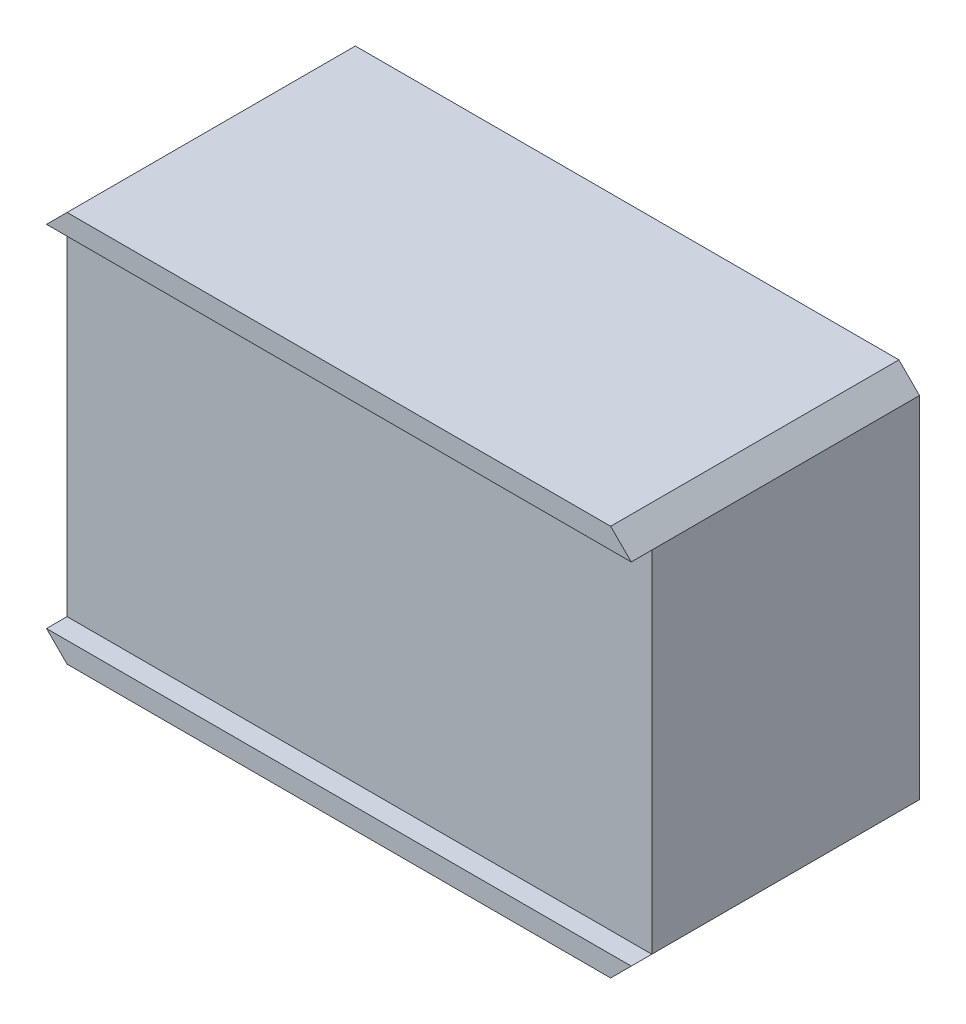
SolidWorks part; units mm, degrees
ref_plane "前视基准面" through (0, 0, 0) normal (0, 0, 1) x (1, 0, 0)
ref_plane "上视基准面" through (0, 0, 0) normal (0, 1, 0) x (1, 0, 0)
ref_plane "右视基准面" through (0, 0, 0) normal (1, 0, 0) x (0, 0, -1)
sketch "草图1" plane through (0, 0, 0) normal (0, 0, 1) x (1, 0, 0)
  line L1 (-28.4, -19) -> (28.4, -19)
  line L2 (-28.4, -19) -> (-28.4, 19)
  line L3 (-28.4, 19) -> (28.4, 19)
  line L4 (28.4, -19) -> (28.4, 19)
  line L5 (-28.4, -19) -> (28.4, 19) construction
  line L6 (-28.4, 19) -> (28.4, -19) construction
  point P0 (0, 0)
  dimension "D1" = 56.8
  dimension "D2" = 38
extrude "凸台-拉伸1" add sketch "草图1" along normal mid plane 28
chamfer "倒角1" distance 2 angle 45 4 edges at (28.4, -19, 0) (-28.4, -19, 0) (-28.4, 19, 0) (28.4, 19, 0)
sketch "草图2" plane through (28.4, 0, 0) normal (1, 0, 0) x (0, 0, -1)
  line L1 (-14, 17) -> (-12, 17)
  line L2 (-14, 17) -> (-14, -17)
  line L3 (-14, -17) -> (-12, -17)
  line L4 (-12, 17) -> (-12, -17)
  line L5 (-14, 17) -> (-14, 19) construction
  line L6 (-14, -17) -> (-14, 17) construction
  point P4 (-12, 0)
  dimension "D1" = 34
  dimension "D2" = 2
extrude "切除-拉伸1" cut sketch "草图2" against normal through all
